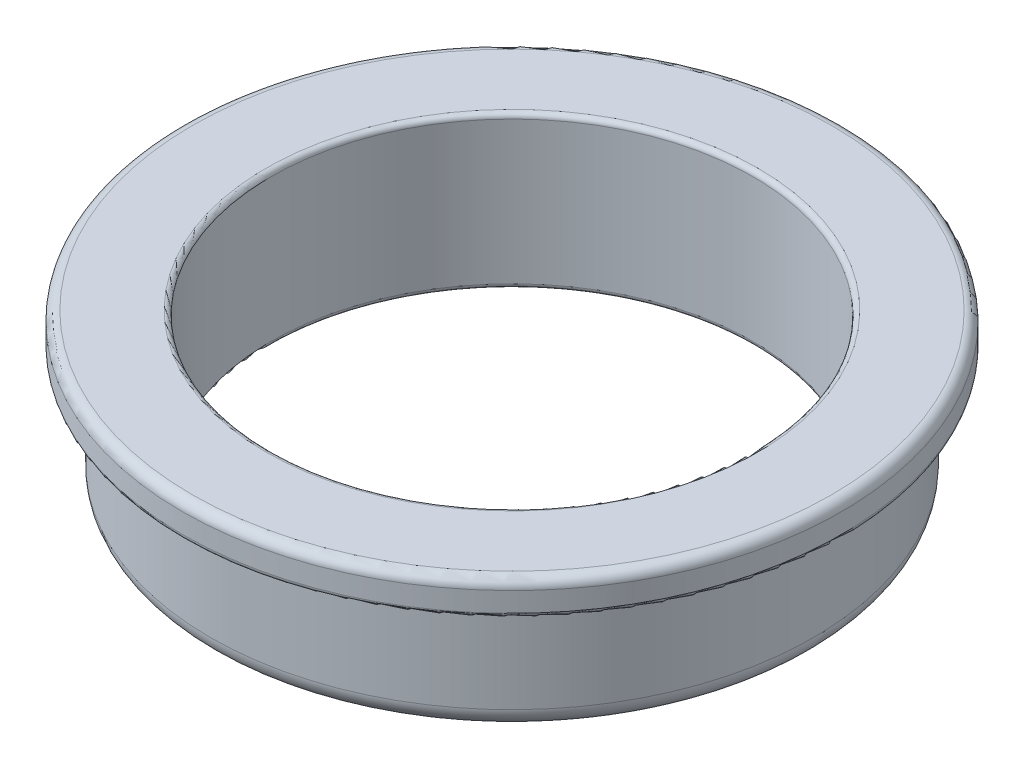
from build123d import *

# Parameters (mm, degrees)
SKETCH1_R           = 30.65
BOSS_EXTRUDE1_DEPTH = 12
SKETCH2_R           = 33.5
BOSS_EXTRUDE2_DEPTH = 3.5
SKETCH3_R           = 24.5
CUT_EXTRUDE1_DEPTH  = 50.847266725
FILLET1_R           = 1
FILLET2_R           = 2
FILLET3_R           = 0.5


with BuildPart() as part:
    # Sketch1 → Boss-Extrude1 (new body)
    with BuildSketch(Plane(origin=(0, 0, 0), x_dir=(1, 0, 0), z_dir=(0, 1, 0))):
        with Locations(Location((0, 0, 0), (0, 0, 270))):
            Circle(SKETCH1_R)
    extrude(amount=-BOSS_EXTRUDE1_DEPTH)

    # Sketch2 → Boss-Extrude2 (add)
    with BuildSketch(Plane(origin=(0, 0, 0), x_dir=(1, 0, 0), z_dir=(0, 1, 0))):
        with Locations(Location((0, 0, 0), (0, 0, 270))):
            Circle(SKETCH2_R)
    extrude(amount=BOSS_EXTRUDE2_DEPTH)

    # Sketch3 → Cut-Extrude1 (cut, through all)
    with BuildSketch(Plane(origin=(0, 3.5, 0), x_dir=(1, 0, 0), z_dir=(0, 1, 0))):
        with Locations(Location((0, 0, 0), (0, 0, 270))):
            Circle(SKETCH3_R)
    extrude(amount=-CUT_EXTRUDE1_DEPTH, mode=Mode.SUBTRACT)

    # Fillet1
    fillet1_edges = [part.edges().sort_by_distance(p)[0] for p in [
        (0, 3.5, -33.5),
    ]]
    fillet(fillet1_edges, radius=FILLET1_R)

    # Fillet2
    fillet2_edges = [part.edges().sort_by_distance(p)[0] for p in [
        (0, -12, -30.65),
    ]]
    fillet(fillet2_edges, radius=FILLET2_R)

    # Fillet3
    fillet3_edges = [part.edges().sort_by_distance(p)[0] for p in [
        (0, -12, -24.5),
        (0, 3.5, -24.5),
        (0, 0, -33.5),
    ]]
    fillet(fillet3_edges, radius=FILLET3_R)


solid = part.part
